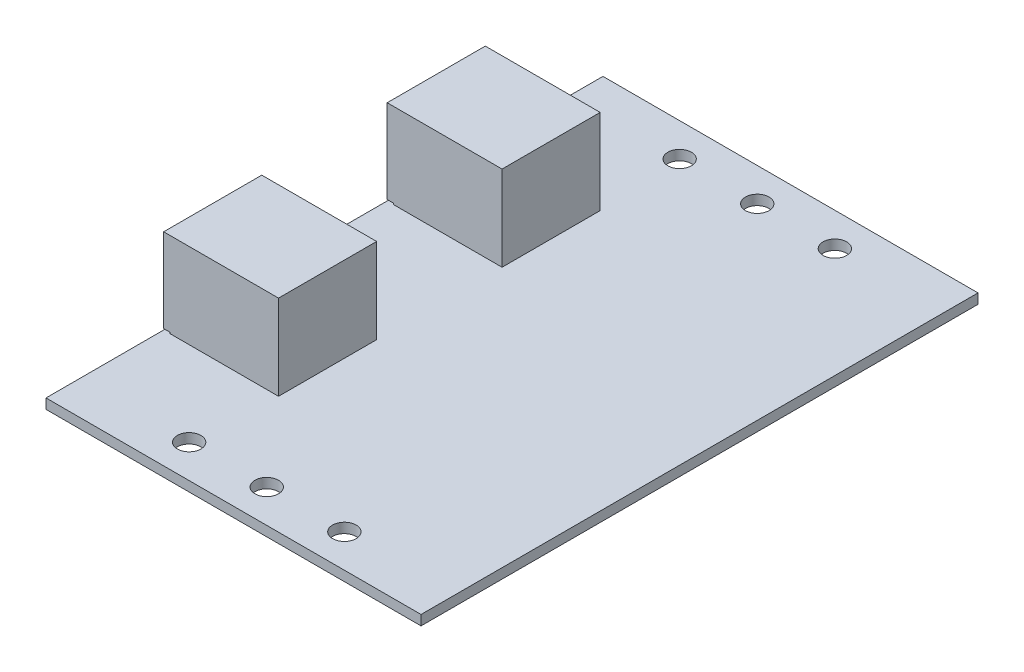
from build123d import *

# Parameters (mm, degrees)
SKETCH_1_W          = 60.4
SKETCH_1_H          = 89.7
EXTRUDE_1_DEPTH     = 1.6
SKETCH_2_R          = 1.9
CUT_EXTRUDE_1_DEPTH = 1.6
SKETCH_3_W          = 15.8
SKETCH_3_H          = 13.7
EXTRUDE_2_DEPTH     = 18.5
SKETCH_4_W          = 51.8
SKETCH_4_H          = 0.2
CUT_EXTRUDE_2_DEPTH = 1
SKETCH_5_W          = 12.792520148
SKETCH_5_H          = 10.634773198
SKETCH_5_W_2        = 12.994853118
SKETCH_5_H_2        = 11.260006872
CUT_EXTRUDE_3_DEPTH = 1


with BuildPart() as part:
    # 草图1 → 凸台-拉伸1 (new body)
    with BuildSketch(Plane(origin=(0, 0, 0), x_dir=(1, 0, 0), z_dir=(0, 1, 0))):
        Rectangle(SKETCH_1_W, SKETCH_1_H)
    extrude(amount=EXTRUDE_1_DEPTH)

    # 草图2 → 切除-拉伸1 (cut)
    with BuildSketch(Plane(origin=(0, 1.6, 0), x_dir=(1, 0, 0), z_dir=(0, 1, 0))):
        with Locations(Location((-12.5, -39.5, 0), (0, 0, 270))):
            Circle(SKETCH_2_R)
        with Locations(Location((12.5, -39.5, 0), (0, 0, 270))):
            Circle(SKETCH_2_R)
        with Locations(Location((-12.5, 39.5, 0), (0, 0, 270))):
            Circle(SKETCH_2_R)
        with Locations(Location((12.5, 39.5, 0), (0, 0, 270))):
            Circle(SKETCH_2_R)
        with Locations(Location((0, 39.5, 0), (0, 0, 270))):
            Circle(SKETCH_2_R)
        with Locations(Location((0, -39.5, 0), (0, 0, 270))):
            Circle(SKETCH_2_R)
    extrude(amount=-CUT_EXTRUDE_1_DEPTH, mode=Mode.SUBTRACT)

    # 草图3 → 凸台-拉伸2 (add)
    with BuildSketch(Plane.ZY.offset(30.2)):
        with Locations((18, 8.45)):
            Rectangle(SKETCH_3_W, SKETCH_3_H)
        with Locations((-18, 8.45)):
            Rectangle(SKETCH_3_W, SKETCH_3_H)
    extrude(amount=-EXTRUDE_2_DEPTH)

    # 草图4 → 切除-拉伸2 (cut)
    with BuildSketch(Plane.ZY.offset(30.2)):
        with Locations((0, 1.7)):
            Rectangle(SKETCH_4_W, SKETCH_4_H)
    extrude(amount=-CUT_EXTRUDE_2_DEPTH, mode=Mode.SUBTRACT)

    # 草图5 → 切除-拉伸3 (cut)
    with BuildSketch(Plane.ZY.offset(30.2)):
        with Locations((18, 8.55)):
            Rectangle(SKETCH_5_W, SKETCH_5_H)
        with Locations((-18, 8.55)):
            Rectangle(SKETCH_5_W_2, SKETCH_5_H_2)
    extrude(amount=-CUT_EXTRUDE_3_DEPTH, mode=Mode.SUBTRACT)


solid = part.part
